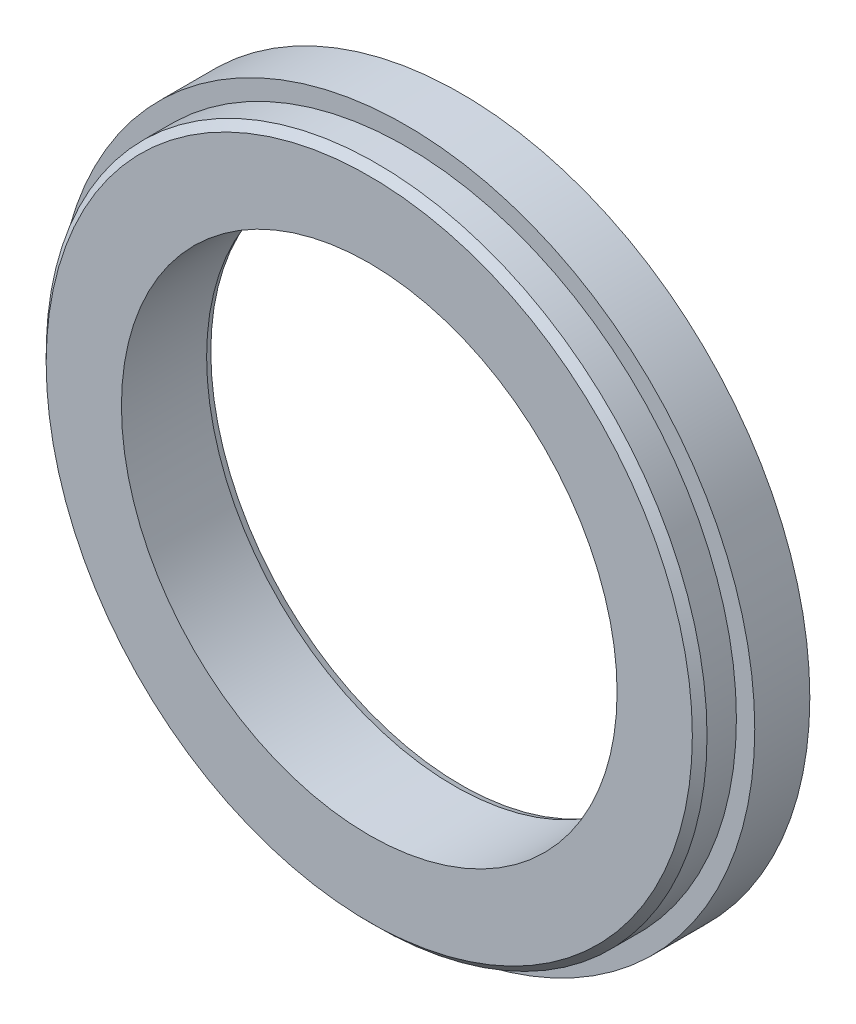
from build123d import *

# Parameters (mm, degrees)
SKETCH1_R                  = 95
SKETCH1_R_2                = 67.5
BOSS_EXTRUDE1_DEPTH        = 15
SKETCH2_R                  = 90
SKETCH2_R_2                = 67.5
BOSS_EXTRUDE2_DEPTH        = 10
CHAMFER1_SIZE              = 2
CHAMFER2_SIZE              = 1.8
CHAMFER2_SIZE2             = 0.655146422
M12X1_5_TAPPED_HOLE1_D     = 10.5
M12X1_5_TAPPED_HOLE1_DEPTH = 20
M12X1_5_TAPPED_HOLE1_TIP   = 3.15451825


with BuildPart() as part:
    # Sketch1 → Boss-Extrude1 (new body)
    with BuildSketch(Plane.XY):
        Circle(SKETCH1_R)
        Circle(SKETCH1_R_2, mode=Mode.SUBTRACT)
    extrude(amount=BOSS_EXTRUDE1_DEPTH)

    # Sketch2 → Boss-Extrude2 (add)
    with BuildSketch(Plane.XY.offset(15)):
        Circle(SKETCH2_R)
        Circle(SKETCH2_R_2, mode=Mode.SUBTRACT)
    extrude(amount=BOSS_EXTRUDE2_DEPTH)

    # Chamfer1
    chamfer1_edges = [part.edges().sort_by_distance(p)[0] for p in [
        (-90, 0, 25),
    ]]
    chamfer(chamfer1_edges, length=CHAMFER1_SIZE)

    # Chamfer2
    chamfer2_edges = [part.edges().sort_by_distance(p)[0] for p in [
        (-67.5, 0, 0),
    ]]
    chamfer2_side = [part.faces().sort_by_distance(p)[0] for p in [
        (-67.5, 0, 12.5),
    ]]
    chamfer(chamfer2_edges, length=CHAMFER2_SIZE, length2=CHAMFER2_SIZE2, reference=chamfer2_side[0])

    # M12x1.5 Tapped Hole1
    with Locations(Plane(origin=(40.25, 69.715045005, 0), x_dir=(-1, 0, 0), z_dir=(0, 0, -1))):
        with Locations((0, 0), (80.5, 0), (120.75, -69.715045005), (80.5, -139.43009001), (-40.25, -69.715045005), (0, -139.43009001)):
            Hole(M12X1_5_TAPPED_HOLE1_D / 2, depth=M12X1_5_TAPPED_HOLE1_DEPTH)
            with Locations((0, 0, -(M12X1_5_TAPPED_HOLE1_DEPTH + M12X1_5_TAPPED_HOLE1_TIP / 2))):  # 118° drill point
                Cone(0, M12X1_5_TAPPED_HOLE1_D / 2, M12X1_5_TAPPED_HOLE1_TIP, mode=Mode.SUBTRACT)


solid = part.part
